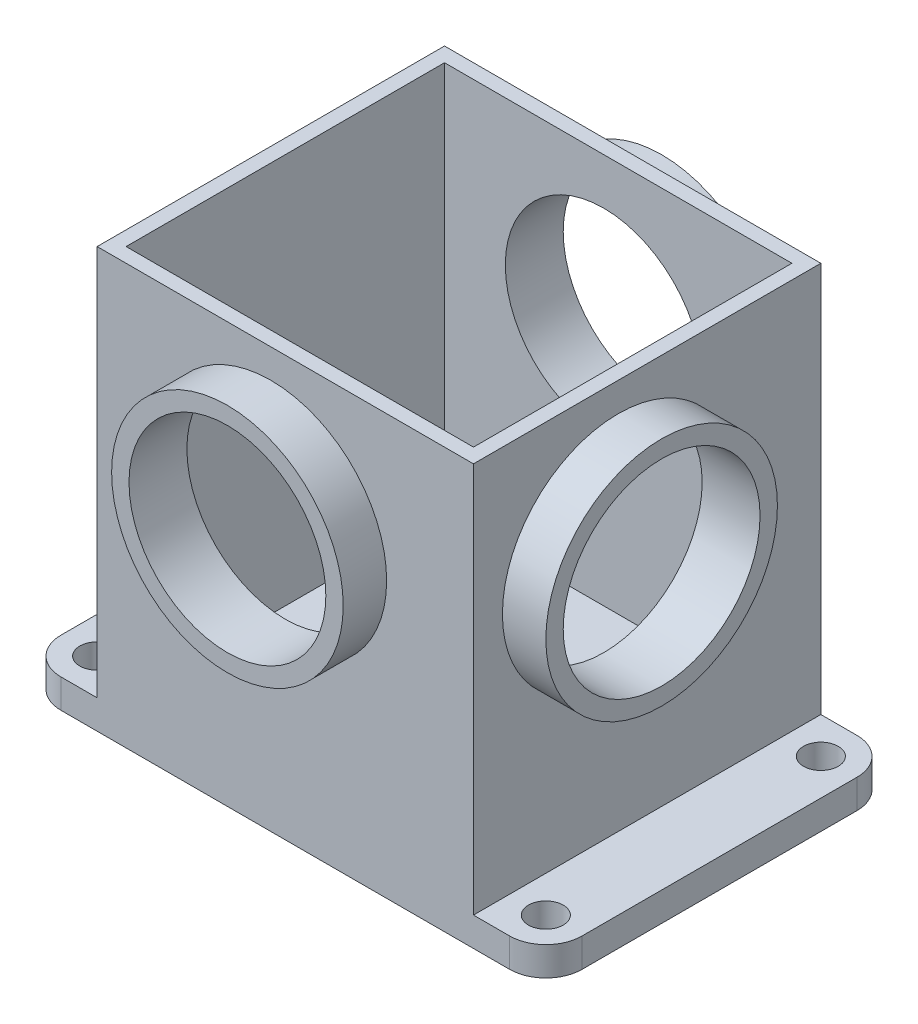
SolidWorks part; units mm, degrees
ref_plane "前视基准面" through (0, 0, 0) normal (0, 0, 1) x (1, 0, 0)
ref_plane "上视基准面" through (0, 0, 0) normal (0, 1, 0) x (1, 0, 0)
ref_plane "右视基准面" through (0, 0, 0) normal (1, 0, 0) x (0, 0, -1)
sketch "草图1" plane through (0, 0, 0) normal (0, 1, 0) x (1, 0, 0)
  line L0 (0, 120) -> (-12.5, 120)
  line L1 (0, 0) -> (130, 0)
  line L3 (0, 120) -> (130, 120)
  line L5 (-25, 107.5) -> (-25, 12.5)
  line L6 (-12.5, 0) -> (0, 0)
  line L7 (130, 0) -> (142.5, 0)
  line L8 (155, 12.5) -> (155, 107.5)
  line L9 (142.5, 120) -> (130, 120)
  arc A0 (155, 107.5) -> (142.5, 120) centre (142.5, 107.5) ccw
  arc A1 (155, 12.5) -> (142.5, 0) centre (142.5, 12.5) cw
  arc A2 (-12.5, 0) -> (-25, 12.5) centre (-12.5, 12.5) cw
  arc A3 (-25, 107.5) -> (-12.5, 120) centre (-12.5, 107.5) cw
  dimension "D1" = 12.5
  dimension "D2" = 12.5
  dimension "D3" = 12.5
  dimension "D5" = 130
extrude "凸台-拉伸1" add sketch "草图1" along normal blind 10
sketch "草图2" plane through (0, 10, 0) normal (0, 1, 0) x (1, 0, 0)
  circle A0 centre (-12.5, 107.5) radius 6
  circle A1 centre (142.5, 107.5) radius 6
  circle A2 centre (142.5, 12.5) radius 6
  circle A3 centre (-12.5, 12.5) radius 6
sketch "草图3" plane through (0, 10, 0) normal (0, 1, 0) x (1, 0, 0)
  line L0 (142.5, 120) -> (-12.5, 120) construction
  line L1 (0, 0) -> (130, 0)
  line L2 (0, 0) -> (0, 120)
  line L3 (0, 120) -> (130, 120)
  line L4 (130, 0) -> (130, 120)
  line L6 (5, 115) -> (125, 115)
  line L7 (5, 115) -> (5, 5)
  line L8 (5, 5) -> (125, 5)
  line L9 (125, 115) -> (125, 5)
  dimension "D1" = 120
  dimension "D2" = 110
  dimension "D3" = 5
  dimension "D4" = 5
extrude "切除-拉伸1" cut sketch "草图2" against normal through all
extrude "凸台-拉伸4" add sketch "草图3" along normal blind 135
sketch "草图4" plane through (0, 0, 0) normal (0, 0, 1) x (1, 0, 0)
  line L0 (-12.5, 10) -> (0, 10) construction
  line L1 (0, 145) -> (0, 10) construction
  circle A0 centre (60, 95) radius 40
  dimension "D1" = 85
  dimension "D2" = 60
extrude "凸台-拉伸5" add sketch "草图4" along normal blind 15
sketch "草图6" plane through (0, 0, 15) normal (0, 0, 1) x (1, 0, 0)
  circle A0 centre (60, 95) radius 34
extrude "切除-拉伸2" cut sketch "草图6" against normal blind 20
sketch "草图7" plane through (130, 0, 0) normal (1, 0, 0) x (0, 0, -1)
  line L0 (0, 10) -> (120, 10) construction
  line L2 (0, 145) -> (0, 10) construction
  circle A0 centre (50, 95) radius 40
  dimension "D1" = 85
  dimension "D2" = 50
extrude "凸台-拉伸6" add sketch "草图7" along normal blind 15
sketch "草图8" plane through (145, 0, 0) normal (1, 0, 0) x (0, 0, -1)
  circle A0 centre (50, 95) radius 34
extrude "切除-拉伸3" cut sketch "草图8" against normal blind 20
sketch "草图9" plane through (0, 0, -120) normal (0, 0, -1) x (-1, 0, 0)
  circle A0 centre (-60, 95) radius 40
extrude "凸台-拉伸7" add sketch "草图9" along normal blind 15
sketch "草图10" plane through (0, 0, -135) normal (0, 0, -1) x (-1, 0, 0)
  circle A0 centre (-60, 95) radius 34
extrude "切除-拉伸4" cut sketch "草图10" against normal blind 20
